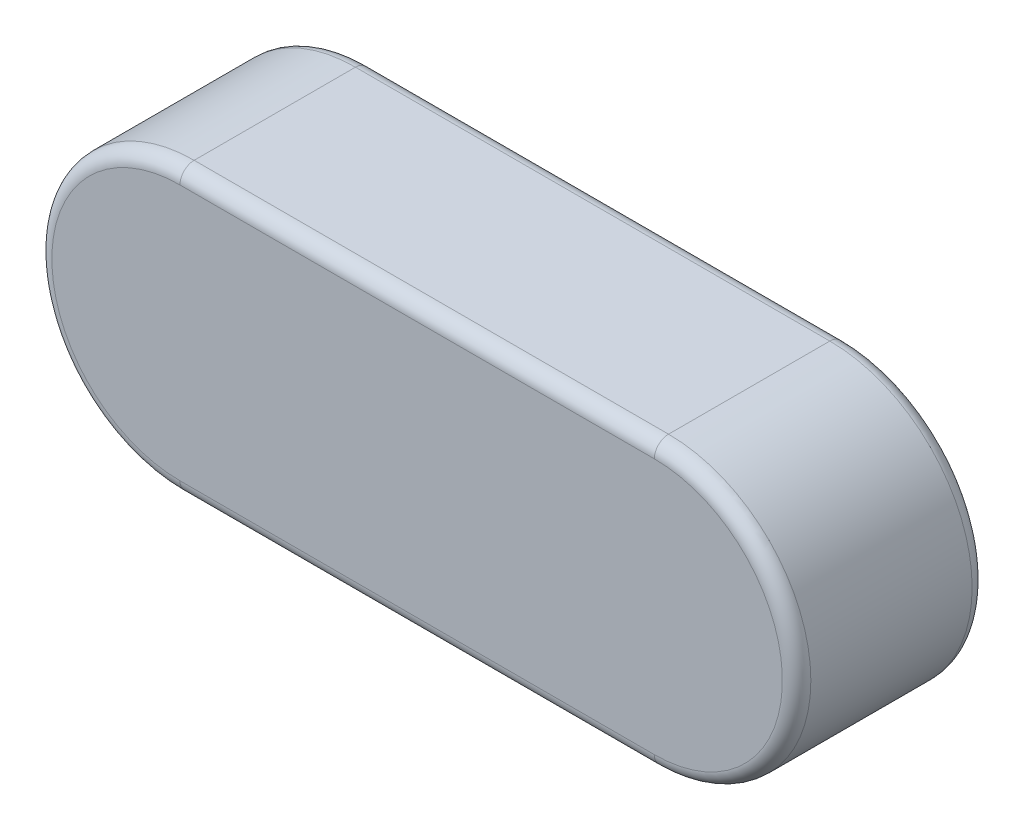
SolidWorks part; units mm, degrees
material "45"
ref_plane "基准面1" through (0, 0, 0) normal (0, 0, 1) x (1, 0, 0)
ref_plane "基准面2" through (0, 0, 0) normal (0, 1, 0) x (1, 0, 0)
ref_plane "基准面3" through (0, 0, 0) normal (1, 0, 0) x (0, 0, -1)
sketch "尺寸草图" plane through (0, 0, 0) normal (0, 0, 1) x (1, 0, 0)
  line L0 (-16, 0) -> (16, 0) construction
  point P3 (-8, 0)
  point P4 (-0.6, 0)
  point P5 (0, 0)
  point P8 (-12, 0)
  point P11 (0, 0)
sketch "草图1" plane through (0, 0, 0) normal (0, 0, 1) x (1, 0, 0)
  line L0 (-28.0599, 0) -> (30.562, 0) construction
  line L1 (-10, 6) -> (10, 6)
  line L2 (-10, -6) -> (10, -6)
  line L3 (0, 2.9108) -> (0, -2.1805) construction
  arc A0 (-10, 6) -> (-10, -6) centre (-10, 0) ccw
  arc A1 (10, 6) -> (10, -6) centre (10, 0) cw
extrude "基体-拉伸" add sketch "草图1" along normal blind 8
fillet "圆角1" radius 0.6 8 edges at (16, 0, 8) (0, 6, 8) (-16, 0, 8) (0, 6, 0) (16, 0, 0) (0, -6, 0) (-16, 0, 0) (0, -6, 8)
equation "\"D3@草图1\" = \"L@尺寸草图\""
equation "\"D1@草图1\" = \"b@尺寸草图\" / 2"
equation "\"D1@圆角1\" = \"r@尺寸草图\""
equation "\"D1@基体-拉伸\" = \"h@尺寸草图\""
